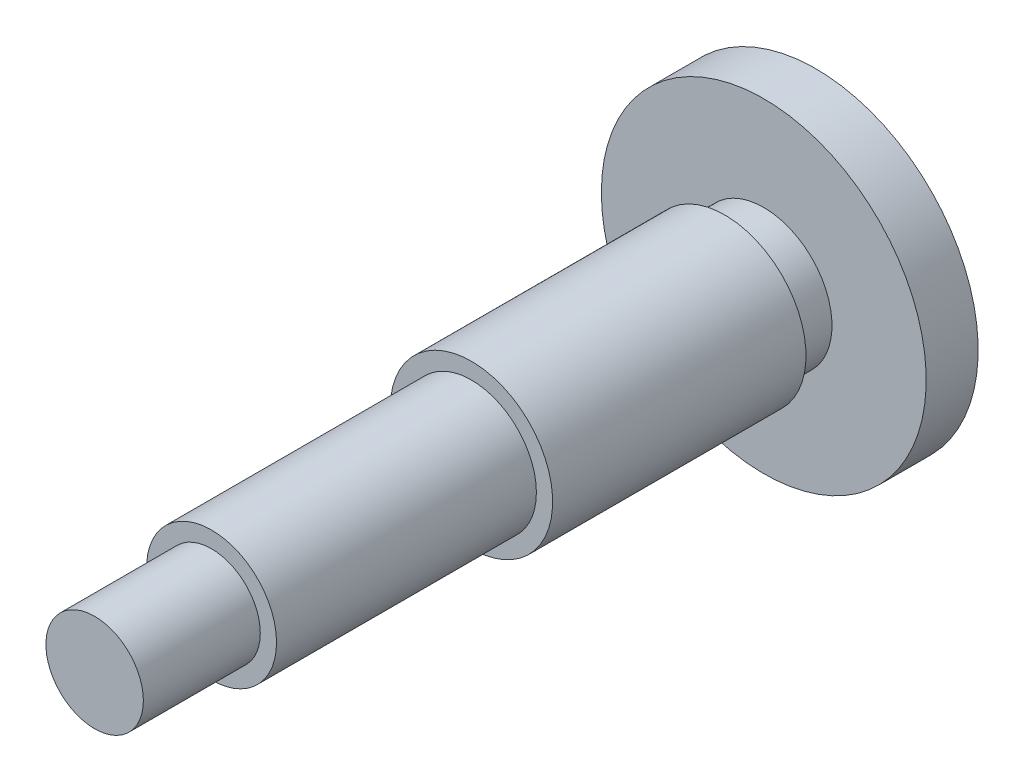
SolidWorks part; units mm, degrees
ref_plane "前视基准面" through (0, 0, 0) normal (0, 0, 1) x (1, 0, 0)
ref_plane "上视基准面" through (0, 0, 0) normal (0, 1, 0) x (1, 0, 0)
ref_plane "右视基准面" through (0, 0, 0) normal (1, 0, 0) x (0, 0, -1)
sketch "草图1" plane through (0, 0, 0) normal (0, 0, 1) x (1, 0, 0)
  circle A0 centre (0, 0) radius 12.5
  dimension "D1" = 25
extrude "凸台-拉伸1" add sketch "草图1" along normal blind 45
cosmetic thread "装饰螺纹线1" parameters "D2"=24
sketch "草图2" plane through (0, 0, 0) normal (0, 0, -1) x (-1, 0, 0)
  circle A0 centre (0, 0) radius 25
  dimension "D1" = 50
extrude "凸台-拉伸2" add sketch "草图2" along normal blind 8
sketch "草图3" plane through (0, 0, 45) normal (0, 0, 1) x (1, 0, 0)
  circle A0 centre (0, 0) radius 10
  dimension "D1" = 20
extrude "凸台-拉伸3" add sketch "草图3" along normal blind 40
sketch "草图5" plane through (0, 0, 0) normal (0, 1, 0) x (1, 0, 0)
  line L0 (12.5, 0) -> (10.5, 0)
  line L1 (10.5, 0) -> (10.5, -6)
  line L2 (10.5, -6) -> (12.5, -6)
  line L3 (12.5, -6) -> (12.5, 0)
  line L4 (0, 0) -> (0, -45) construction
  line L5 (-10, -45) -> (10, -45) construction
  dimension "D1" = 6
  dimension "D2" = 2
revolve "切除-旋转1" cut sketch "草图5" angle 360 about L4
sketch "草图6" plane through (0, 0, 85) normal (0, 0, 1) x (1, 0, 0)
  circle A0 centre (0, 0) radius 7.5
  dimension "D1" = 15
extrude "凸台-拉伸4" add sketch "草图6" along normal blind 18
